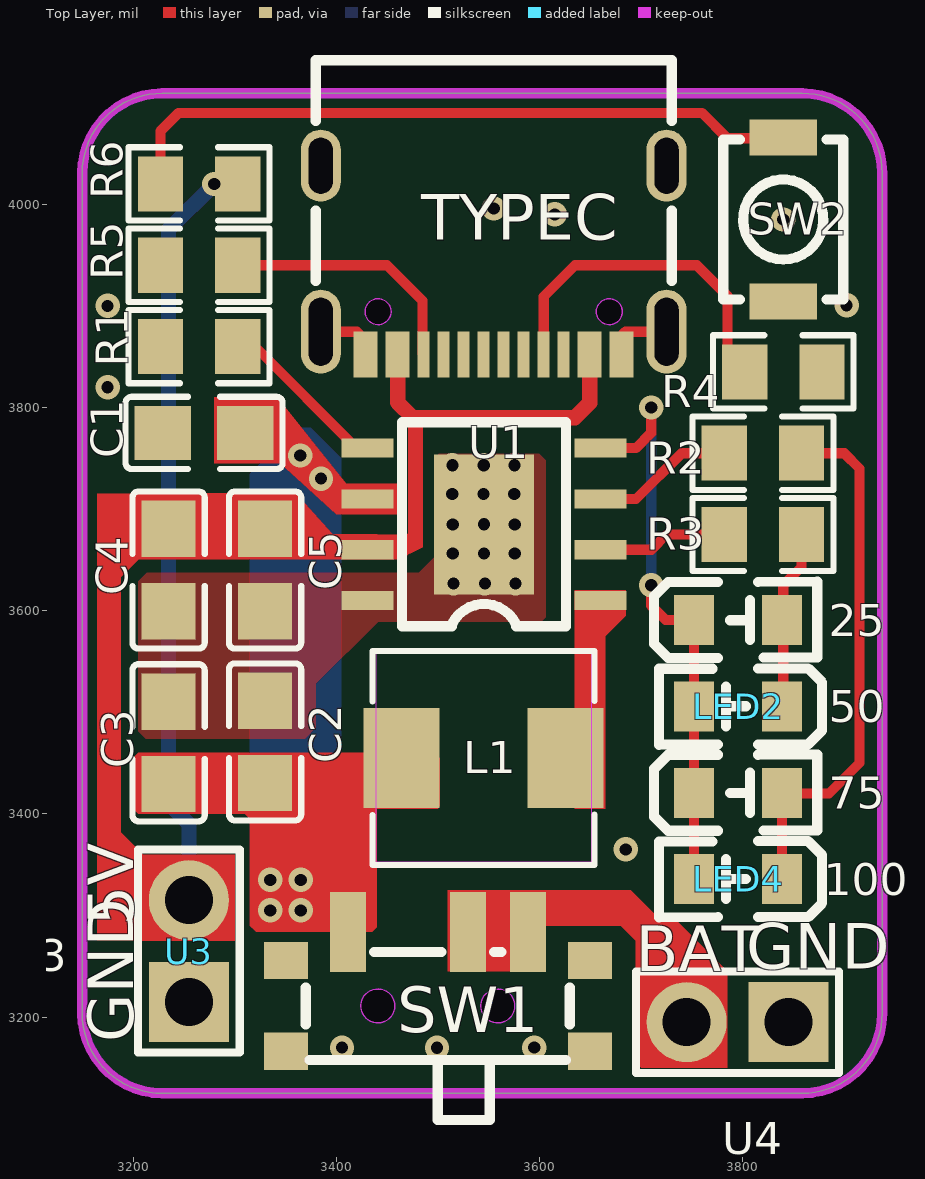
[diagram p0: Top Layer view]
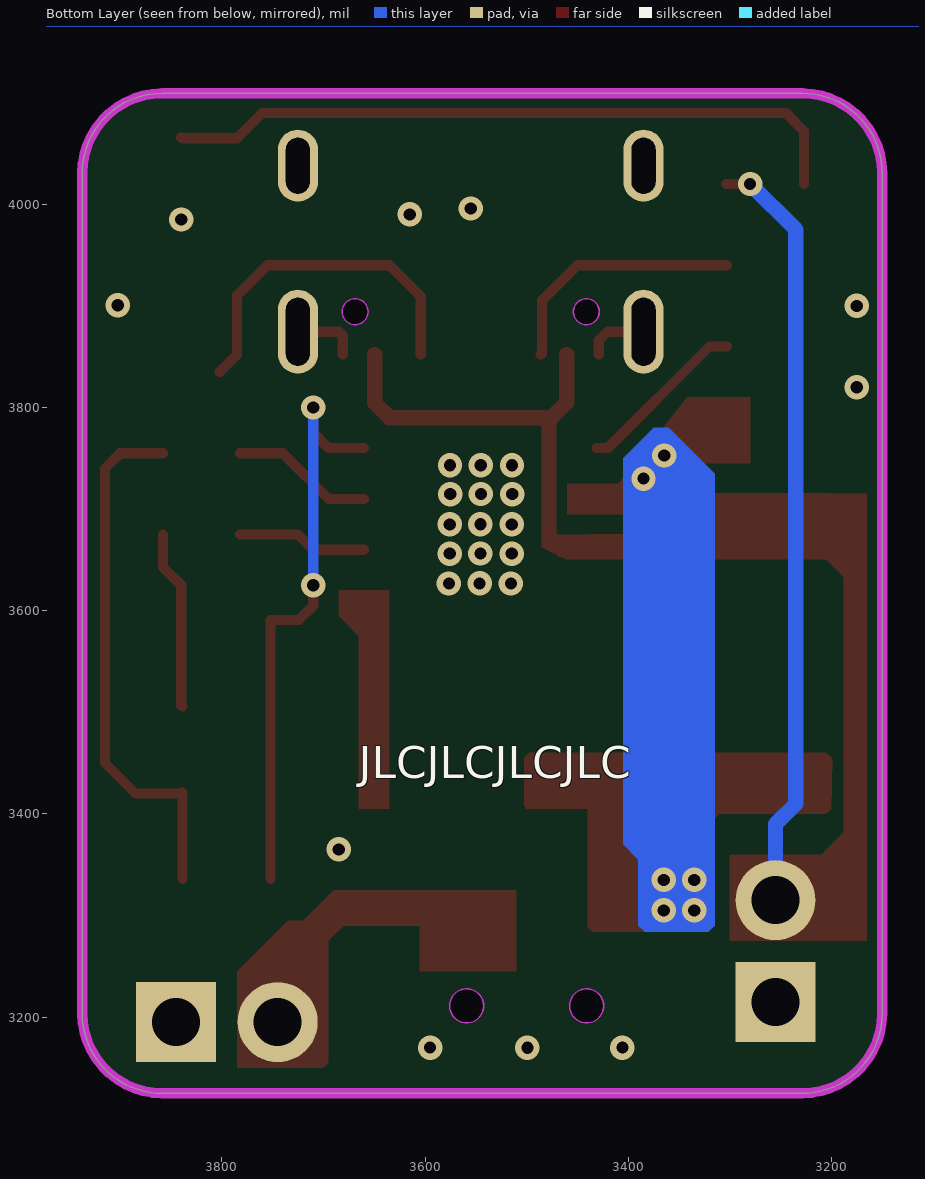
[diagram p1: Bottom Layer view, seen from below]
# Altium PCB MISC51179.pcbdoc
Units mil, origin at the board's own origin, x right, y up, seen from the top; angles counter-clockwise.
Board outline 787.4 x 984.25 mil, 2 copper layers (Top Layer, Bottom Layer), stack 62.205 mil thick; 22 components, 14 nets, 70 pads, 34 vias.

## Layer stack, top to bottom
Top Solder Mask Layer: solder mask 0.394, Dk 3.3
Top Layer: signal copper 1.378
Dielectric1: surface 59.449, FR4, Dk 4.5
Bottom Layer: signal copper 1.378
Bottom Solder Mask Layer: solder mask 0.394, Dk 3.3

## Board outline
3228.74,4109.25 ccw(c3228.74,4030.51) 3150,4030.51 3150,3203.74 ccw(c3228.74,3203.74) 3228.74,3125 3858.66,3125 ccw(c3858.66,3203.74) 3937.4,3203.74 3937.4,4030.51 ccw(c3858.66,4030.51) 3858.66,4109.25 3228.74,4109.25

## Design rules (kind name [scope] priority, off if disabled: settings)
BoardOutlineClearance Plane_innerPlane_1 [All] p2 off: genericclearance=6 ignorepadtopadclearanceinfootprint=FALSE except(0: Arc-SplitContinuation Track-SplitContinuation SMDPad-SplitContinuation THPad-SplitContinuation Via-SplitContinuation Fill-SplitContinuation Region-SplitContinuation Poly-SplitContinuation Text-SplitContinuation Hole-SplitContinuation; 6: Arc-CutoutEdge Track-CutoutEdge SMDPad-CutoutEdge THPad-CutoutEdge Via-CutoutEdge Fill-CutoutEdge Region-CutoutEdge Text-CutoutEdge Hole-CutoutEdge; 10: Poly-OutlineEdge Poly-CutoutEdge; 11.8: Arc-OutlineEdge Track-OutlineEdge SMDPad-OutlineEdge THPad-OutlineEdge Via-OutlineEdge Fill-OutlineEdge Region-OutlineEdge Text-OutlineEdge Hole-OutlineEdge)
BoardOutlineClearance Copper_copperRegion_1 [All] p4 off: genericclearance=6 ignorepadtopadclearanceinfootprint=FALSE except(0: Arc-SplitContinuation Track-SplitContinuation SMDPad-SplitContinuation THPad-SplitContinuation Via-SplitContinuation Fill-SplitContinuation Region-SplitContinuation Poly-SplitContinuation Text-SplitContinuation Hole-SplitContinuation; 6: Arc-CutoutEdge Track-CutoutEdge SMDPad-CutoutEdge THPad-CutoutEdge Via-CutoutEdge Fill-CutoutEdge Region-CutoutEdge Text-CutoutEdge Hole-CutoutEdge; 10: Poly-OutlineEdge Poly-CutoutEdge; 11.8: Arc-OutlineEdge Track-OutlineEdge SMDPad-OutlineEdge THPad-OutlineEdge Via-OutlineEdge Fill-OutlineEdge Region-OutlineEdge Text-OutlineEdge Hole-OutlineEdge)
BoardOutlineClearance safeClearance_1 [All] p6: genericclearance=6 ignorepadtopadclearanceinfootprint=FALSE except(0: Arc-SplitContinuation Track-SplitContinuation SMDPad-SplitContinuation THPad-SplitContinuation Via-SplitContinuation Fill-SplitContinuation Region-SplitContinuation Poly-SplitContinuation Text-SplitContinuation Hole-SplitContinuation; 6: Arc-CutoutEdge Track-CutoutEdge SMDPad-CutoutEdge THPad-CutoutEdge Via-CutoutEdge Fill-CutoutEdge Region-CutoutEdge Text-CutoutEdge Hole-CutoutEdge; 10: Poly-OutlineEdge Poly-CutoutEdge; 11.8: Arc-OutlineEdge Track-OutlineEdge SMDPad-OutlineEdge THPad-OutlineEdge Via-OutlineEdge Fill-OutlineEdge Region-OutlineEdge Text-OutlineEdge Hole-OutlineEdge)
Clearance Plane_innerPlane [All] p1 off: gap=6 ignorepadtopadclearanceinfootprint=FALSE except(10: Poly-Track Poly-SMDPad Poly-THPad Poly-Via Poly-Fill Poly-Region Poly-Poly Poly-Arc Poly-Text Poly-Hole)
Clearance Copper_copperRegion [All] p3 off: gap=6 ignorepadtopadclearanceinfootprint=FALSE except(10: Poly-Track Poly-SMDPad Poly-THPad Poly-Via Poly-Fill Poly-Region Poly-Poly Poly-Arc Poly-Text Poly-Hole)
Clearance safeClearance [All] p5: gap=6 ignorepadtopadclearanceinfootprint=FALSE except(10: Poly-Track Poly-SMDPad Poly-THPad Poly-Via Poly-Fill Poly-Region Poly-Poly Poly-Arc Poly-Text Poly-Hole)
DiffPairsRouting differentialPair [All] p1: maxlimit=6 minlimit=6 mostfreqgap=6 toplayer_minwidth=5 toplayer_prefwidth=10 toplayer_maxwidth=100 toplayer_mingap=6 toplayer_prefgap=6 toplayer_maxgap=6 bottomlayer_minwidth=5 bottomlayer_prefwidth=10 bottomlayer_maxwidth=100 bottomlayer_mingap=6 bottomlayer_prefgap=6 bottomlayer_maxgap=6 maxuncoupledlength=10
HoleToHoleClearance otherClearance [All] p1: gap=11.8 allowstackedmicrovias=TRUE
Length netLength [All] p1: minlimit=0 maxlimit=0
PasteMaskExpansion pasteMaskExpansion [All] p1: expansion=0
PlaneConnect innerPlane [All] p1: planeconnectstyle=Relief reliefexpansion=20 reliefentries=4 reliefconductorwidth=10 reliefairgap=10
PolygonConnect copperRegion [All] p1: connectstyle=Relief reliefconductorwidth=10 reliefentries=4 polygonreliefangle="90 Angle" airgapwidth=10 via.connectstyle=Relief via.reliefconductorwidth=10 via.reliefentries=4 via.polygonreliefangle="90 Angle" via.airgapwidth=10
RoutingVias viaSize [All] p1: holewidth=12.01 width=24.02 viastyle="Through Hole" minholewidth=11.81 minwidth=19.68 maxholewidth=236.22 maxwidth=393.7
SolderMaskExpansion solderMaskExpansion [IsVia] p1: expansion=-1000 istentingtop=TRUE
SolderMaskExpansion solderMaskExpansion [All] p2: expansion=4 istentingtop=FALSE
Width trackWidth [All] p1: maxlimit=100 minlimit=5 preferedwidth=10

## Components (designator, comment, footprint, x,y, rotation, side; value= is the part's Value field where it differs from the comment)
C1 "1uF" C0805 3270,3775 r180 top
C2 "22uF" C0805 3330,3470.9 r270 top
C3 "22uF" C0805 3235,3470 r270 top
C4 "22uF" C0805 3235,3640 r90 top
C5 "22uF" C0805 3330,3640 r90 top
L1 "2.2uH" IND-SMD_L5.4-W5.2 3545,3455 r0 top
LED1 "led0805" LED0805-RD 3795.55,3590.79 r0 top
LED2 "led0805" LED0805-RD 3795.55,3505.79 r180 top
LED3 "led0805" LED0805-RD 3795.55,3420.79 r0 top
LED4 "led0805" LED0805-RD 3795.55,3335.79 r180 top
R1 "75KΩ" R0805 3265,3860 r0 top
R2 "1kΩ" R0805 3820,3755 r180 top
R3 "1kΩ" R0805 3820,3675 r180 top
R4 "5.1KΩ" R0805 3840,3835 r180 top
R5 "5.1KΩ" R0805 3265,3940 r0 top
R6 "51Ω" R0805 3265,4020 r180 top
SW1 "MK-12C02-G015" SW-SMD_G-SWITCH_MK-12C02-G015 3500,3225 r0 top
SW2 "ST-1185U" SW-SMD_ST-1185U 3840,3985 r270 top
TYPEC "TYPE-C 16PIN 3MD(385)" USB-C-SMD_TYPE-C16PIN 3555,3945 r180 top
U1 "ETA9740" ESOP-8 3545,3685 r180 top
U3 "2.54-1*2" HDR-TH_2P-P2.54-V-M 3255,3265 r90 top
U4 "2.54-1*2" HDR-TH_2P-P2.54-V-M 3795,3195 r180 top

## Footprints (in the part's own frame and the unit in brackets; to place one, negate y for a bottom-side part, rotate by r counter-clockwise, add the part's x,y. Pads: shape width x height; smd on the part's side, far side on the other; paste and mask are expansions set on the pad)
C0805 [mm]
  rect 1.41x1.35 smd paste-100 mask+0.051: 1(-1.03,0) 2(1.03,0)
  silkscreen extent -1.96,-0.9 1.96,0.9
ESOP-8 [mil]
  rect 51.18x18.9 smd paste+0 mask+4: 1(-115,75) 2(-115,25) 3(-115,-25) 4(-115,-75) 5(114,-75) 6(114,-25) 7(114,25) 8(114,75)
  rect 98.42x137.79 smd paste+0 mask+4: 9(-0.5,0)
  silkscreen extent -81,-100 80,100
HDR-TH_2P-P2.54-V-M [mm]
  rect 2x2 hole 1.2 paste+0 mask+0.051: 1(-1.27,0)
  round 2 hole 1.2 paste+0 mask+0.051: 2(1.27,0)
  silkscreen extent -2.54,-1.27 2.54,1.27
IND-SMD_L5.4-W5.2 [mm]
  rect 1.9x2.5 smd paste+0 mask+0.051: 1(2.05,0) 2(-2.05,0)
  silkscreen extent -2.78,-2.68 2.78,2.68
LED0805-RD [mm]
  rect 1x1.25 smd paste+0 mask+0.051: 1(-1.1,0) 2(1.1,0)
  silkscreen extent -2.1,-0.95 1.98,0.96
R0805 [mil]
  rect 44.59x54.21 smd paste-3937.01 mask+2: 1(-38.04,0) 2(38.04,0)
  silkscreen extent -69,-36 69,36
SW-SMD_G-SWITCH_MK-12C02-G015 [mm]
  rect 0.9x2 smd paste+0 mask+0.051: 1(-2.25,1.491) 2(0.75,1.491) 3(2.25,1.491)
  rect 1.1x0.93 smd paste+0 mask+0.051: 4(3.8,0.779) 5(3.8,-1.491) 6(-3.8,-1.491) 7(-3.8,0.779)
  Board Outline Layer circle w0.003: c1.5,-0.356 r0.425
  Board Outline Layer circle w0.003: c-1.5,-0.356 r0.425
  Board Outline Layer region: 1.925,-0.356 1.883,-0.54 1.765,-0.688 1.595,-0.77 1.405,-0.77 1.235,-0.688 1.117,-0.54 1.075,-0.356 1.075,-0.356 1.117,-0.171 1.235,-0.023 1.405,0.059 1.595,0.059 1.765,-0.023 1.883,-0.171 1.925,-0.356
  Board Outline Layer region: 1.925,-0.356 1.916,-0.444 1.888,-0.528 1.844,-0.605 1.784,-0.671 1.712,-0.724 1.631,-0.76 1.544,-0.778 1.456,-0.778 1.369,-0.76 1.287,-0.724 1.216,-0.671 1.156,-0.605 1.112,-0.528 1.084,-0.444 1.075,-0.356 1.084,-0.267 1.112,-0.183 1.156,-0.106 1.216,-0.04 1.287,0.012 1.369,0.049 1.456,0.067 1.544,0.067 1.631,0.049 1.712,0.012 1.784,-0.04 1.844,-0.106 1.888,-0.183 1.916,-0.267
  Board Outline Layer region: -1.075,-0.356 -1.117,-0.54 -1.235,-0.688 -1.405,-0.77 -1.595,-0.77 -1.765,-0.688 -1.883,-0.54 -1.925,-0.356 -1.925,-0.356 -1.883,-0.172 -1.765,-0.024 -1.595,0.058 -1.405,0.058 -1.235,-0.024 -1.117,-0.172 -1.075,-0.356
  Board Outline Layer region: -1.075,-0.356 -1.084,-0.444 -1.112,-0.529 -1.156,-0.606 -1.216,-0.672 -1.288,-0.724 -1.369,-0.76 -1.456,-0.779 -1.544,-0.779 -1.631,-0.76 -1.713,-0.724 -1.784,-0.672 -1.844,-0.606 -1.888,-0.529 -1.916,-0.444 -1.925,-0.356 -1.916,-0.268 -1.888,-0.183 -1.844,-0.106 -1.784,-0.04 -1.713,0.012 -1.631,0.048 -1.544,0.067 -1.456,0.067 -1.369,0.048 -1.288,0.012 -1.216,-0.04 -1.156,-0.106 -1.112,-0.183 -1.084,-0.268
  Multi-Layer board cut-out: 1.925,-0.356 1.883,-0.54 1.765,-0.688 1.595,-0.77 1.405,-0.77 1.235,-0.688 1.117,-0.54 1.075,-0.356 1.075,-0.356 1.117,-0.171 1.235,-0.023 1.405,0.059 1.595,0.059 1.765,-0.023 1.883,-0.171 1.925,-0.356
  Multi-Layer board cut-out: -1.075,-0.356 -1.117,-0.54 -1.235,-0.688 -1.405,-0.77 -1.595,-0.77 -1.765,-0.688 -1.883,-0.54 -1.925,-0.356 -1.925,-0.356 -1.883,-0.172 -1.765,-0.024 -1.595,0.058 -1.405,0.058 -1.235,-0.024 -1.117,-0.172 -1.075,-0.356
  silkscreen extent -3.3,-3.21 3.3,0.99
SW-SMD_ST-1185U [mil]
  rect 35.4x66.9 smd paste+0 mask+2: 1(-80.7,0) 2(80.7,0)
  silkscreen extent -79,-59 79,59
USB-C-SMD_TYPE-C16PIN [mil]
  oval 39.4x82.7 hole 23.6 slot 66.9 at 90 deg paste+0 mask+2: 1(-170.1,70.4) 2(170.1,70.4)
  oval 39.4x70.9 hole 23.6 slot 55.1 at 90 deg paste+0 mask+2: 3(-170.1,-93) 4(170.1,-93)
  rect 23.6x45.3 smd paste-3937.01 mask+2: A1B12(-126,93) A4B9(-94.5,93) B1A12(126,93) B4A9(94.5,93)
  rect 11.8x45.3 smd paste-3937.01 mask+2: A5(-49.2,93) A6(-9.8,93) A7(9.8,93) A8(-68.9,93) B5(68.9,93) B6(29.5,93) B7(-29.5,93) B8(49.2,93)
  Board Outline Layer circle w0.1: c113.8,50.7 r12.8
  Board Outline Layer circle w0.1: c-113.8,50.7 r12.8
  Board Outline Layer region: 101,50.7 102.27,56.25 105.82,60.71 110.95,63.18 116.65,63.18 121.78,60.71 125.33,56.25 126.6,50.7 126.6,50.7 125.33,45.15 121.78,40.69 116.65,38.22 110.95,38.22 105.82,40.69 102.27,45.15 101,50.7
  Board Outline Layer region: 101,50.7 101.37,53.76 102.47,56.65 104.22,59.19 106.53,61.23 109.26,62.67 112.26,63.41 115.34,63.41 118.34,62.67 121.07,61.23 123.38,59.19 125.13,56.65 126.23,53.76 126.6,50.7 126.23,47.64 125.13,44.75 123.38,42.21 121.07,40.17 118.34,38.73 115.34,37.99 112.26,37.99 109.26,38.73 106.53,40.17 104.22,42.21 102.47,44.75 101.37,47.64
  Board Outline Layer region: -126.6,50.7 -125.33,56.25 -121.78,60.71 -116.65,63.18 -110.95,63.18 -105.82,60.71 -102.27,56.25 -101,50.7 -101,50.7 -102.27,45.15 -105.82,40.69 -110.95,38.22 -116.65,38.22 -121.78,40.69 -125.33,45.15 -126.6,50.7
  Board Outline Layer region: -126.6,50.7 -126.23,53.76 -125.13,56.65 -123.38,59.19 -121.07,61.23 -118.34,62.67 -115.34,63.41 -112.26,63.41 -109.26,62.67 -106.53,61.23 -104.22,59.19 -102.47,56.65 -101.37,53.76 -101,50.7 -101.37,47.64 -102.47,44.75 -104.22,42.21 -106.53,40.17 -109.26,38.73 -112.26,37.99 -115.34,37.99 -118.34,38.73 -121.07,40.17 -123.38,42.21 -125.13,44.75 -126.23,47.64
  Multi-Layer board cut-out: 101,50.7 102.27,56.25 105.82,60.71 110.95,63.18 116.65,63.18 121.78,60.71 125.33,56.25 126.6,50.7 126.6,50.7 125.33,45.15 121.78,40.69 116.65,38.22 110.95,38.22 105.82,40.69 102.27,45.15 101,50.7
  Multi-Layer board cut-out: -126.6,50.7 -125.33,56.25 -121.78,60.71 -116.65,63.18 -110.95,63.18 -105.82,60.71 -102.27,56.25 -101,50.7 -101,50.7 -102.27,45.15 -105.82,40.69 -110.95,38.22 -116.65,38.22 -121.78,40.69 -125.33,45.15 -126.6,50.7
  silkscreen extent -175,-197 175,20

## Via types
v1: diameter 24.02, hole 12, Top Layer to Bottom Layer, 34 vias

## Nets (pads, with @x,y where several pads share a name; then routed paths per layer and width w, separated by ;. In a path a pad name is that pad's centre, name@x,y a point inside that pad or via, vN(x,y) a via of type N, cw(c..) or ccw(c..) an arc to the next point about the centre after c; other vN are vias at no path point)
$1N2660: LED1.2 LED2.1 R3.1 | length 177.2
  Top Layer w10: LED2.1 3840,3506.92 3840,3625 3858.04,3643.04 R3.1
$1N2785: LED3.2 LED4.1 R2.1 | length 527.1
  Top Layer w10: LED4.1 LED3.2 3839.65,3420 3885,3420 3915,3450 3915,3740 3900,3755 R2.1
$1N17245: L1.1 U1.1
$1N17288: R3.2 U1.2 | length 128.2
  Top Layer w10: U1.2 3710,3660 3725,3675 R3.2
$1N17330: R2.2 U1.3 | length 140.6
  Top Layer w10: U1.3 3695,3710 3740,3755 R2.2
$1N17374: LED1.1 LED2.2 LED3.1 LED4.2 U1.4 | length 579.3
  Top Layer w10: U1.4 3695,3760 3710,3775 v1(3710,3800) ; v1(3710,3625) 3710,3605 3724.21,3590.79 LED1.1 LED2.2 LED3.1 LED4.2
  Bottom Layer w10: v1(3710,3625) v1(3710,3800)
$1N17470: R1.2 U1.5 | length 169.4
  Top Layer w10: R1.2 3320,3860 3420,3760 U1.5
$1N17516: C1.1 C2.2 C3.2 L1.2 SW1.1 U1.6
  other v1: 3335,3305 3365,3305 3335,3335 3365,3335 3385,3730 3364.53,3752.79
$1N18547: R6.2 SW2.1 | length 683.1
  Top Layer w10: R6.2 3226.96,4071.96 3245,4090 3760,4090 3785,4065 3839.3,4065 SW2.1
$1N20218: R5.2 TYPEC.B5 | length 249.9
  Top Layer w10: R5.2 3450,3940 3485,3905 3485,3853.1 TYPEC.B5
$1N20241: R4.2 TYPEC.A5 | length 345.2
  Top Layer w10: TYPEC.A5 3604.2,3909.2 3635,3940 3755,3940 3785,3910 3785,3851.96 R4.2
+5V: C4.2 C5.2 R6.1 TYPEC.A4B9 TYPEC.B4A9 U1.7 U3.2 | length 1221.2
  Top Layer w10: v1(3280,4020) R6.1
  Top Layer w15: U1.7 3465,3660 3477.97,3672.97 3477.97,3787.38 3475.35,3790 ; TYPEC.B4A9 3460.5,3804.85 3475.35,3790 ; TYPEC.A4B9 3649.5,3804.5 3635,3790 3475.35,3790
  Bottom Layer w15: U3.2 3255,3390 3235,3410 3235,3975 v1(3280,4020)
BAT: SW1.2 SW1.3 U4.2
GND: C1.2 C2.1 C3.1 C4.1 C5.1 R1.1 R4.1 R5.1 SW1.4 SW1.5 SW1.6 SW1.7 SW2.2 TYPEC.1 TYPEC.2 TYPEC.3 TYPEC.4 TYPEC.A1B12 TYPEC.B1A12 U1.8 U1.9 U3.1 U4.1 | length 126.3
  Top Layer w10: TYPEC.2 3420.4,3874.6 3429,3866 TYPEC.B1A12 ; TYPEC.A1B12 3681,3871 3684.6,3874.6 TYPEC.1
  other v1: 3405.7,3170 3499.21,3169.76 3595,3170 3685,3365 3515.46,3626.77 3546.29,3626.83 3576.45,3626.77 3514.66,3656.23 3545.5,3656.29 3575.66,3656.23 3514.66,3684.94 3545.5,3685 3575.66,3684.94 3514.2,3714.79 3545.04,3714.85 3575.2,3714.79 3514.4,3743.18 3545.23,3743.23 3575.39,3743.18 3175,3820 3175,3900 3902.37,3900.64 3840,3985 3615,3990 3555,3995.84
pads on no net: TYPEC.A6 TYPEC.A7 TYPEC.A8 TYPEC.B6 TYPEC.B7 TYPEC.B8

## Polygon pours and split planes (outlines as drawn)
GND on Top Layer (solid, remove dead copper, pour order 2): 3025,4150 3025,3000 4050,3000 4050,4150
GND on Bottom Layer (solid, remove dead copper, pour order 2): 3000,4175 3000,3045 4000,3045 4000,4175

## Keep-outs
Top Layer:
  region: 3438.7,3557.38 3438.7,3352.68 3651.3,3352.68 3651.3,3557.38
Board Outline Layer:
  the board outline again, w10

## Other copper
Top Layer:
  region net $1N17516: 3205,3460 3497.22,3460 3502.12,3455.11 3502.12,3407.88 3500,3405 3440,3405 3440,3288.25 3435.64,3283.89 3321.11,3283.89 3315,3290 3315,3395 3310,3400 3205,3400 3199.94,3405.06 3199.37,3454.14
  region net BAT: 3510,3325 3510,3245 3605,3245 3605,3290 3680,3290 3695,3275 3695,3155 3700,3150 3785,3150 3785,3245 3735,3295 3720.59,3295 3717.59,3297.99 3717.01,3297.99 3690,3325
  region net $1N17245: 3685,3620 3685,3595 3665,3575 3665,3405 3635,3405 3635,3620
  region net +5V: 3360.32,3715.49 3201.52,3715.94 3201.52,3650.44 3460,3650 3485,3662.5 3485,3674.9 3396.06,3675.49
  region net $1N17516: 3460,3695 3400,3695 3345,3745 3280,3745 3280,3810 3340.73,3810 3341.31,3810.57 3410,3725 3460,3725
  region net +5V: 3295,3275 3165,3275 3165,3715 3201.73,3715 3210.43,3706.31 3210.43,3655.43 3188.05,3633.05 3188.05,3381.95 3210,3360 3300,3360 3300,3275 3290,3275
Bottom Layer:
  region net $1N17516: 3321.11,3283.89 3315,3290 3315,3735 3360,3780 3375,3780 3405,3750 3405,3370 3390,3355 3390,3290 3383.89,3283.89

## Silkscreen, mask and mechanical layers (free items; w line width, h text height)
Top Silkscreen Layer:
  text "25" at 3885,3575 h31.5
  text "50" at 3885,3490 h31.5
  text "75" at 3885,3405 h31.5
  text "100" at 3880,3320 h31.5
  text "5V" at 3200,3290 h45 r90
  text "GND" at 3803.35,3247.5 h45
  text "BAT" at 3695,3245 h45
  text "GND" at 3200,3175 h45 r90
Bottom Silkscreen Layer:
  text "JLCJLCJLCJLC" at 3665,3435 h31.5